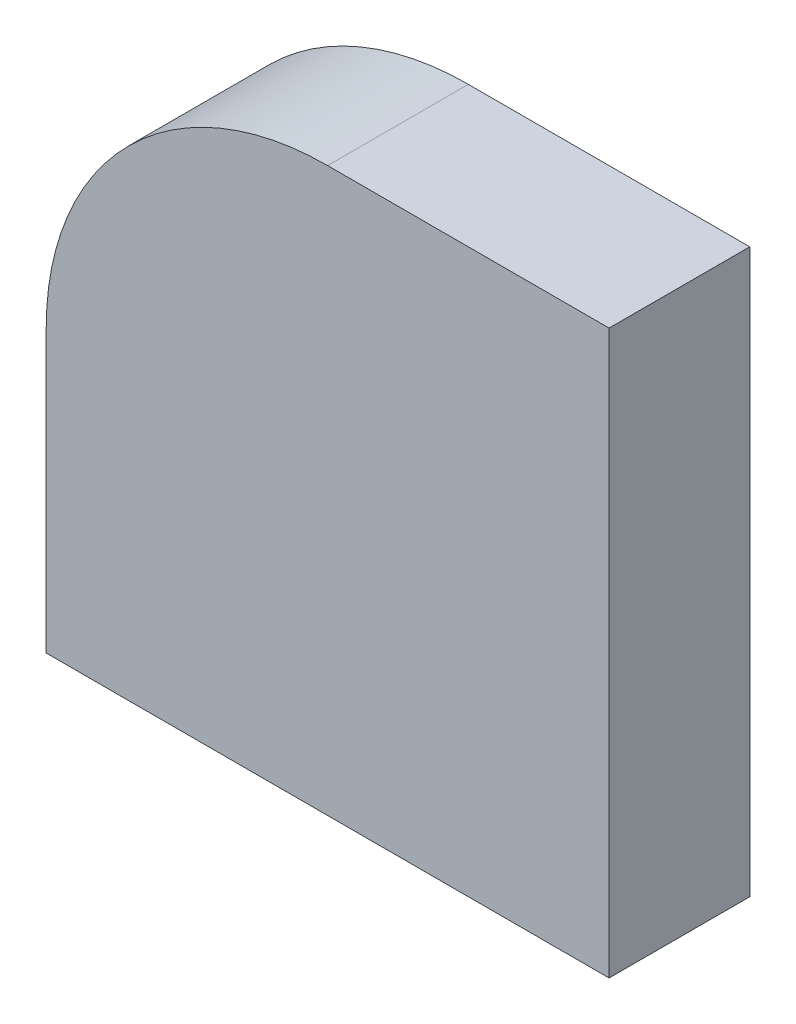
from build123d import *

# Parameters (mm, degrees)
SKETCH1_W           = 40
SKETCH1_H           = 40
BOSS_EXTRUDE1_DEPTH = 10
FILLET1_R           = 20


with BuildPart() as part:
    # Sketch1 → Boss-Extrude1 (new body)
    with BuildSketch(Plane.XY):
        with Locations((20, 20)):
            Rectangle(SKETCH1_W, SKETCH1_H)
    extrude(amount=BOSS_EXTRUDE1_DEPTH)

    # Fillet1
    fillet1_edges = [part.edges().sort_by_distance(p)[0] for p in [
        (0, 40, 5),
    ]]
    fillet(fillet1_edges, radius=FILLET1_R)


solid = part.part
